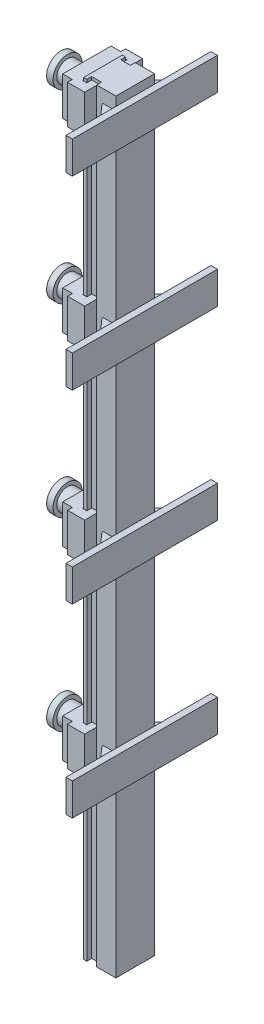
SolidWorks part; units mm, degrees
ref_plane "Front Plane" through (0, 0, 0) normal (0, 0, 1) x (1, 0, 0)
ref_plane "Top Plane" through (0, 0, 0) normal (0, 1, 0) x (1, 0, 0)
ref_plane "Right Plane" through (0, 0, 0) normal (1, 0, 0) x (0, 0, -1)
other "Configuration Table"
sketch "Sketch1" plane through (0, 0, 0) normal (0, 1, 0) x (1, 0, 0)
  line L0 (10, 0) -> (10, -15)
  line L1 (0, 0) -> (10, 0)
  line L2 (0, 0) -> (0, -120)
  line L3 (0, -120) -> (10, -120)
  line L4 (100, 0) -> (100, -120)
  line L5 (10, -15) -> (40, -15)
  line L6 (40, -15) -> (40, 0)
  line L7 (10, -120) -> (10, -105)
  line L8 (10, -105) -> (40, -105)
  line L9 (40, -105) -> (40, -120)
  line L10 (40, 0) -> (100, 0)
  line L11 (40, -120) -> (100, -120)
  dimension "D1" = 100
  dimension "D2" = 120
  dimension "D3" = 10
  dimension "D4" = 15
  dimension "D5" = 15
  dimension "D6" = 30
  dimension "D7" = 30
extrude "Boss-Extrude1" add sketch "Sketch1" along normal blind 2330
sketch "Sketch2" plane through (0, 2330, 0) normal (0, 1, 0) x (1, 0, 0)
  line L0 (60, -120) -> (100, -120)
  line L2 (100, -120) -> (100, 0)
  line L3 (100, 0) -> (60, 0)
  line L4 (100, 0) -> (40, 0) construction
  line L6 (95, 43) -> (95, 60)
  line L7 (95, 60) -> (110, 60)
  line L8 (110, 60) -> (110, -180)
  line L9 (110, -180) -> (95, -180)
  line L10 (95, -180) -> (95, -163)
  line L12 (40, -120) -> (100, -120) construction
  line L13 (95, -163) -> (60, -123)
  line L14 (60, -123) -> (60, -120)
  line L15 (60, 0) -> (60, 3)
  line L16 (60, 3) -> (95, 43)
  dimension "D1" = 40
  dimension "D2" = 40
  dimension "18" = 40
  dimension "D3" = 40
  dimension "D4" = 3
  dimension "D5" = 3
  dimension "D6" = 15
  dimension "D7" = 60
  dimension "D8" = 60
  dimension "D9" = 15
  dimension "D10" = 10
extrude "Boss-Extrude2" add sketch "Sketch2" against normal blind 6
pattern_linear "LPattern1" count 2 spacing 50 along (0, -1, 0) of "Boss-Extrude2"
sketch "Sketch3" plane through (0, 2280, 0) normal (0, 1, 0) x (1, 0, 0)
  line L1 (-55, 0) -> (55, 0) construction
  line L4 (60, 3) -> (98, 3)
  line L5 (98, 3) -> (98, 60)
  line L6 (98, 60) -> (110, 60)
  line L7 (110, 60) -> (110, 0)
  line L8 (110, -180) -> (110, 60) construction
  line L10 (95, 60) -> (95, 43) construction
  line L11 (95, 60) -> (95, 43) construction
  line L13 (60, 3) -> (60, 0)
  line L14 (60, 0) -> (110, 0)
  dimension "D1" = 3
extrude "Boss-Extrude3" add sketch "Sketch3" along normal blind 50
ref_plane "Plane1" through (0, 0, 60) normal (0, 0, 1) x (1, 0, 0)
mirror "Mirror1" about plane through (0, 0, 60) normal (0, 0, 1) of "Boss-Extrude3"
sketch "Sketch4" plane through (0, 0, -3) normal (0, 0, -1) x (-1, 0, 0)
  line L0 (-60, 2302) -> (-98, 2302) construction
  line L3 (-60, 2324) -> (-60, 2280) construction
  line L4 (-98, 2324) -> (-98, 2280) construction
  circle A0 centre (-79, 2302) radius 17.5
  dimension "D1" = 35
extrude "Boss-Extrude4" add sketch "Sketch4" along normal blind 2
sketch "Sketch5" plane through (0, 0, -5) normal (0, 0, -1) x (-1, 0, 0)
  line L1 (-65.5228, 2294.0584) -> (-65.3838, 2309.7008)
  line L2 (-65.3838, 2309.7008) -> (-78.861, 2317.6424)
  line L3 (-78.861, 2317.6424) -> (-92.4772, 2309.9416)
  line L4 (-92.4772, 2309.9416) -> (-92.6162, 2294.2992)
  line L5 (-92.6162, 2294.2992) -> (-79.139, 2286.3576)
  line L6 (-79.139, 2286.3576) -> (-65.5228, 2294.0584)
  circle A0 centre (-79, 2302) radius 13.5472 construction
extrude "Boss-Extrude5" add sketch "Sketch5" along normal blind 12
pattern_linear "LPattern2" count 4 spacing 575 along (0, -1, 0) of "Boss-Extrude5", "Boss-Extrude4", "Mirror1", "Boss-Extrude3", "Boss-Extrude2", "LPattern1"
ref_plane "Plane2" through (0, 2302, 0) normal (0, 1, 0) x (1, 0, 0)
sketch "Sketch6" plane through (0, 2302, 0) normal (0, 1, 0) x (1, 0, 0)
  line L0 (33.1291, 30) -> (33.1291, -13.2917)
  line L2 (33.1291, -13.2917) -> (11.5688, -13.2917)
  line L3 (33.1291, 30) -> (-20, 30)
  line L4 (-20, 30) -> (-20, 15)
  line L5 (-20, 15) -> (-50, 15)
  line L6 (-50, 15) -> (-50, -135)
  line L7 (-50, -135) -> (-20, -135)
  line L8 (-20, -135) -> (-20, -150)
  line L9 (-20, -150) -> (33.1291, -150)
  line L10 (11.5688, -13.2917) -> (11.5688, 2.4469)
  line L11 (11.5688, 2.4469) -> (-1.3688, 2.4469)
  line L12 (-1.3688, 2.4469) -> (-1.3688, -121.6957)
  line L13 (-1.3688, -121.6957) -> (11.5688, -121.6957)
  line L14 (11.5688, -121.6957) -> (11.5688, -106.1654)
  line L15 (11.5688, -106.1654) -> (33.1291, -106.1654)
  line L16 (33.1291, -106.1654) -> (33.1291, -150)
  line L17 (0, -120) -> (10, -120) construction
  line L18 (10, 0) -> (0, 0) construction
  line L19 (0, 0) -> (0, -120) construction
  line L20 (110, -180) -> (110, 60) construction
  dimension "D1" = 30
  dimension "D2" = 30
  dimension "D3" = 20
  dimension "D4" = 20
  dimension "D5" = 15
  dimension "D6" = 15
  dimension "D7" = 160
extrude "Boss-Extrude6" add sketch "Sketch6" along normal blind 60 and the other way blind 60 separate body
sketch "Sketch7" plane through (110, 0, 0) normal (1, 0, 0) x (0, 0, -1)
  line L0 (-180, 2330) -> (60, 2274) construction
  line L2 (-285, 2352) -> (165, 2352)
  line L3 (-285, 2352) -> (-285, 2252)
  line L4 (-285, 2252) -> (165, 2252)
  line L5 (165, 2352) -> (165, 2252)
  line L6 (-285, 2352) -> (165, 2252) construction
  line L7 (-285, 2252) -> (165, 2352) construction
  point P4 (-60, 2302)
  dimension "D1" = 450
  dimension "D2" = 100
extrude "Boss-Extrude7" add sketch "Sketch7" along normal blind 20
sketch "Sketch8" plane through (0, 2330, 0) normal (0, 1, 0) x (1, 0, 0)
  line L0 (0, 0) -> (10, 0)
  line L1 (10, 0) -> (10, -15)
  line L2 (10, -15) -> (40, -15)
  line L3 (40, -15) -> (40, 0)
  line L4 (40, 0) -> (100, 0)
  line L5 (0, 0) -> (0, -120)
  line L6 (0, -120) -> (10, -120)
  line L7 (10, -120) -> (10, -105)
  line L8 (10, -105) -> (40, -105)
  line L9 (40, -105) -> (40, -120)
  line L10 (40, -120) -> (100, -120)
  line L11 (100, -120) -> (100, 0)
  dimension "D1" = 100
extrude "Boss-Extrude8" add sketch "Sketch8" along normal blind 40
pattern_linear "LPattern5" count 4 spacing 575 along (0, -1, 0) of "Boss-Extrude6", "Boss-Extrude7"
sketch "Sketch10" plane through (-50, 0, 0) normal (-1, 0, 0) x (0, 0, 1)
  line L0 (27.5, 2302) -> (-27.5, 2302) construction
  line L1 (60, -33) -> (60, 33) construction
  circle A0 centre (60, 2302) radius 33.5132
  circle A1 centre (60, 1727) radius 33.5132
  circle A2 centre (60, 1152) radius 33.5132
  circle A3 centre (60, 577) radius 33.5132
  dimension "D1" = 4
extrude "Boss-Extrude9" add sketch "Sketch10" along normal blind 60
sketch "Sketch11" plane through (-110, 0, 0) normal (-1, 0, 0) x (0, 0, 1)
  circle A0 centre (60, 2302) radius 45
  circle A1 centre (60, 1727) radius 45
  circle A2 centre (60, 1152) radius 45
  circle A3 centre (60, 577) radius 45
  dimension "D1" = 90
extrude "Boss-Extrude10" add sketch "Sketch11" along normal blind 20
